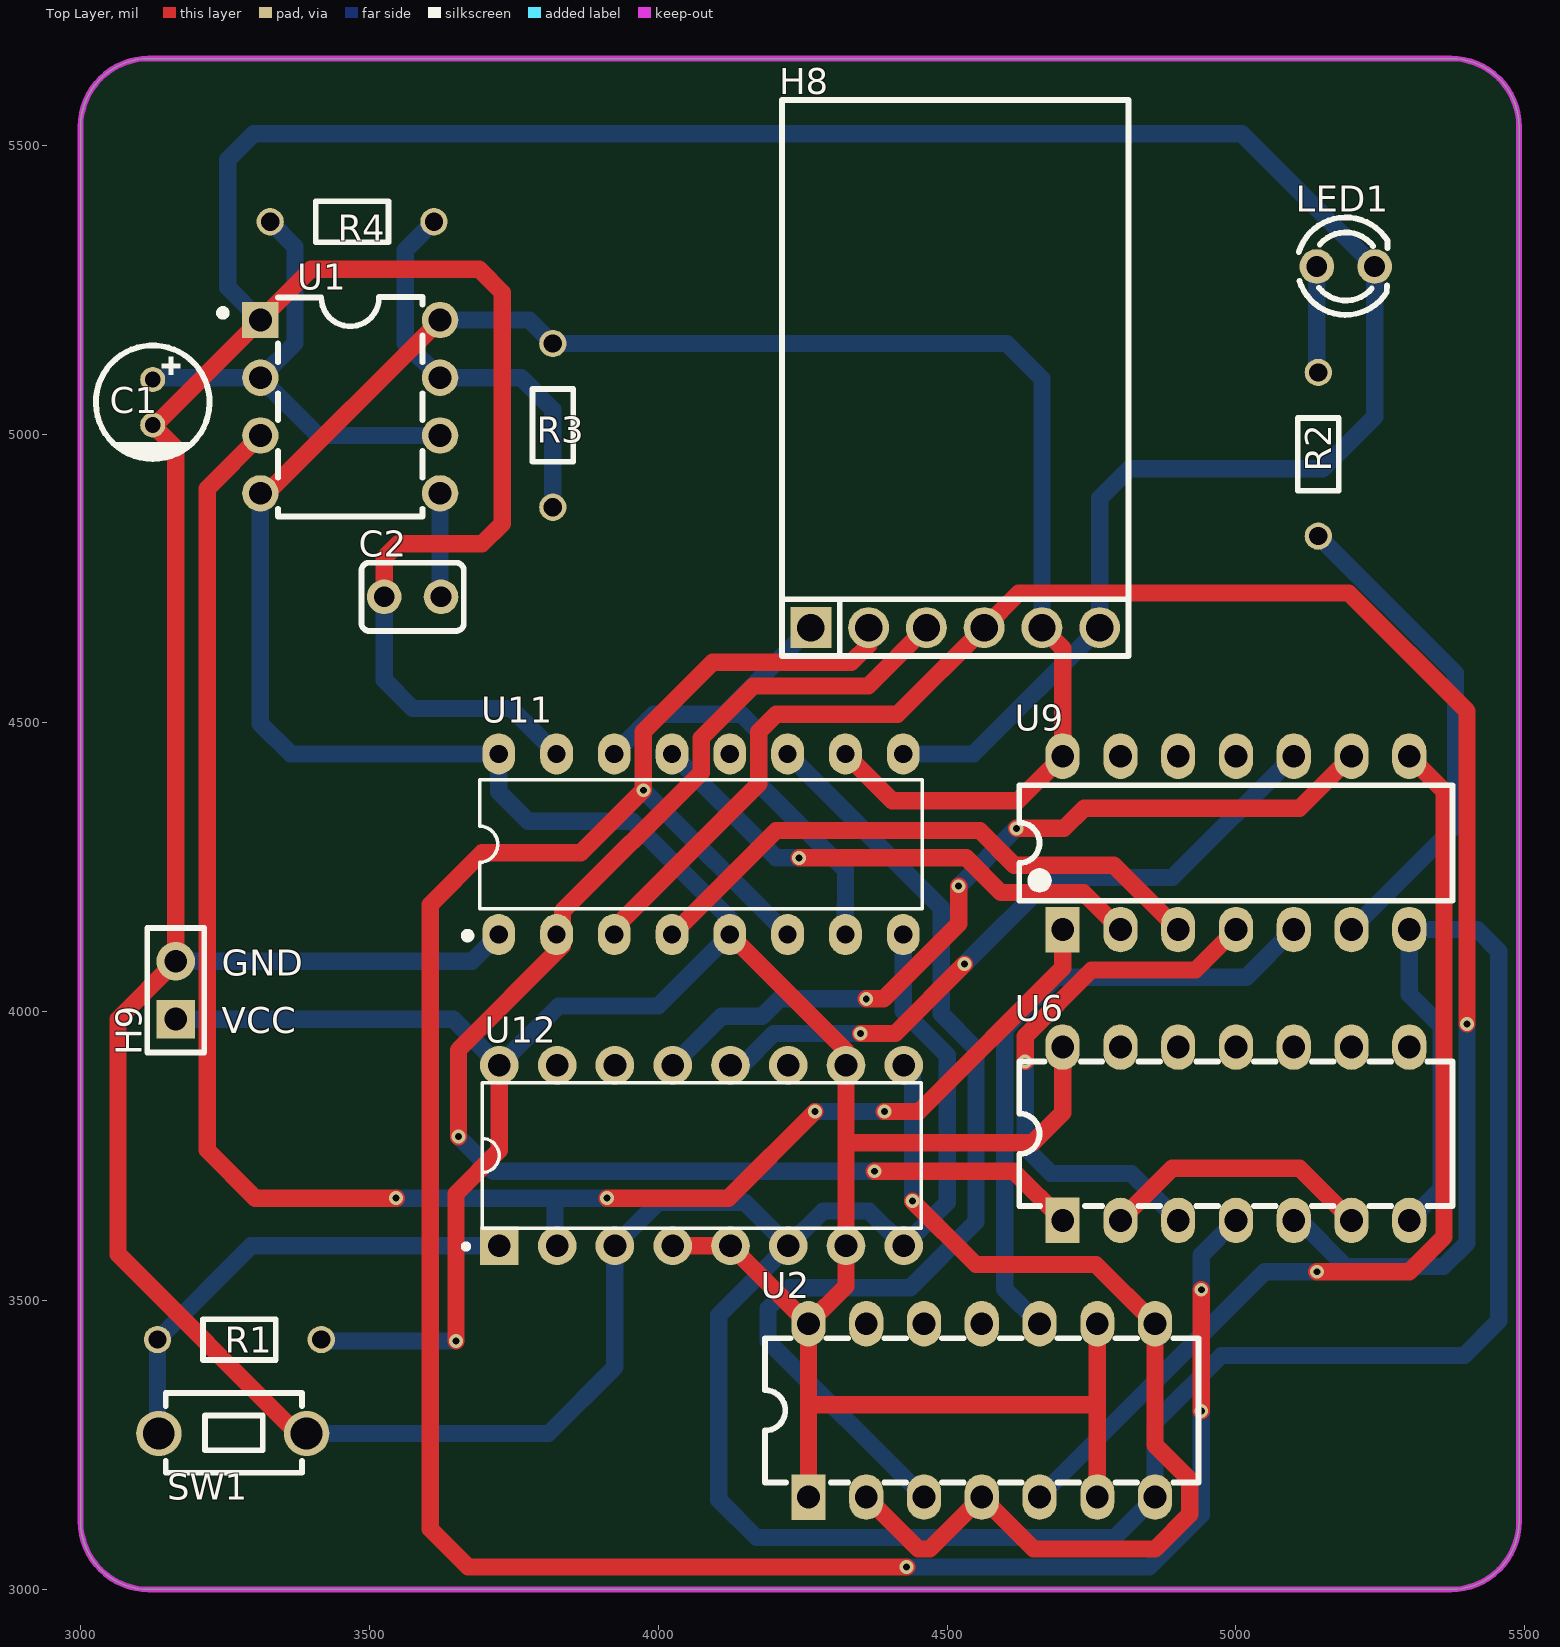
[diagram p0: Top Layer view]
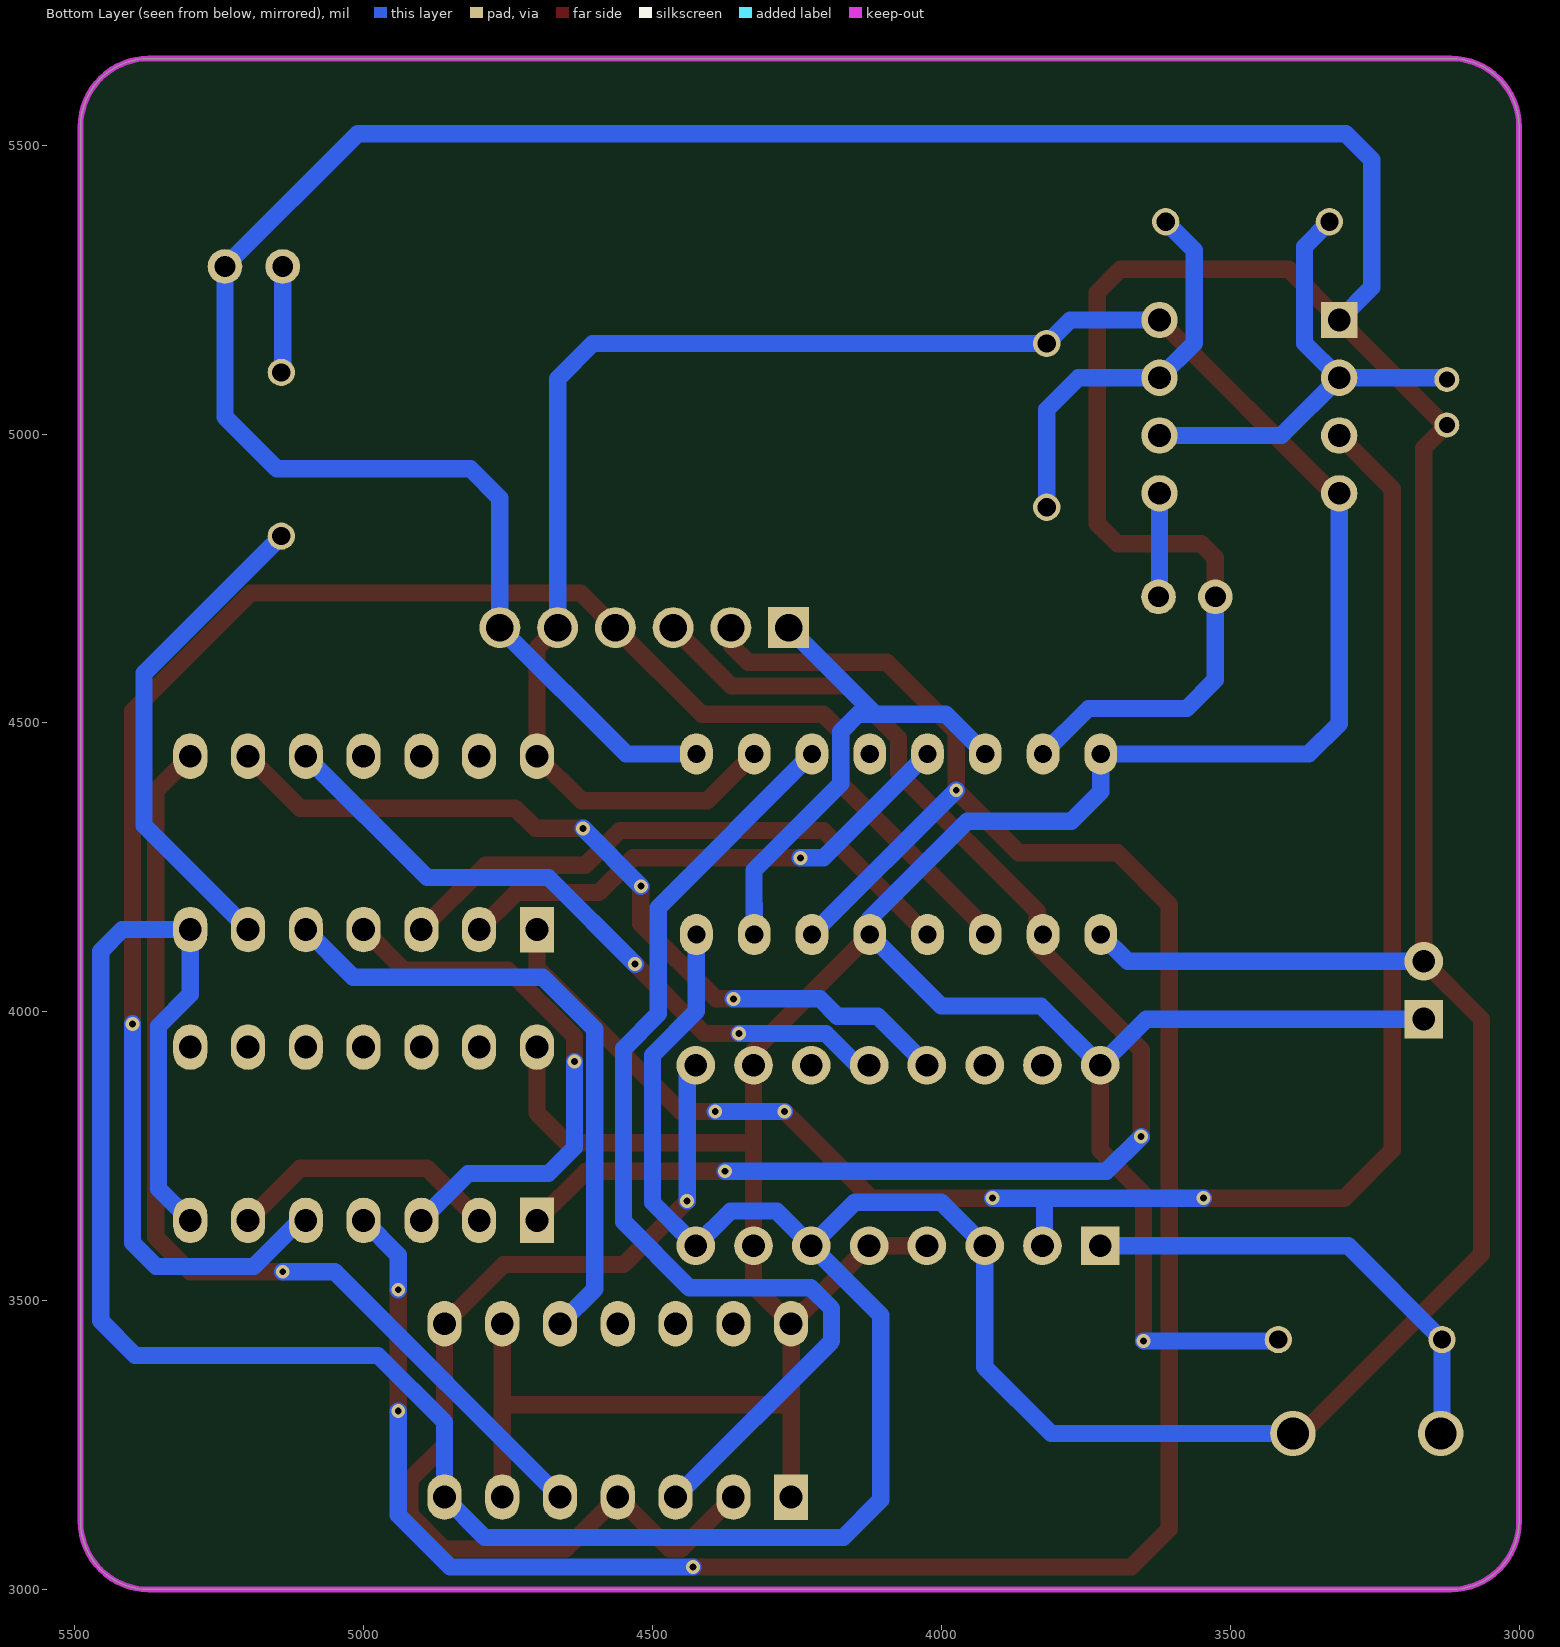
[diagram p1: Bottom Layer view, seen from below]
# Altium PCB MISC51493.pcbdoc
Units mil, origin at the board's own origin, x right, y up, seen from the top; angles counter-clockwise.
Board outline 2490 x 2650 mil, 2 copper layers (Top Layer, Bottom Layer), stack 62.206 mil thick; 16 components, 23 nets, 106 pads, 21 vias.

## Layer stack, top to bottom
Top Solder Mask Layer: solder mask 0.394, Dk 3.3
Top Layer: signal copper 1.379
Dielectric1: surface 59.449, FR4, Dk 4.5
Bottom Layer: signal copper 1.378
Bottom Solder Mask Layer: solder mask 0.394, Dk 3.3

## Board outline
3118.11,5650 ccw(c3118.11,5531.89) 3000,5531.89 3000,3118.11 ccw(c3118.11,3118.11) 3118.11,3000 5371.89,3000 ccw(c5371.89,3118.11) 5490,3118.11 5490,5531.89 ccw(c5371.89,5531.89) 5371.89,5650

## Design rules (kind name [scope] priority, off if disabled: settings)
BoardOutlineClearance copperThickness2oz_1 [All] p2 off: genericclearance=8 ignorepadtopadclearanceinfootprint=FALSE except(0: Arc-SplitContinuation Track-SplitContinuation SMDPad-SplitContinuation THPad-SplitContinuation Via-SplitContinuation Fill-SplitContinuation Region-SplitContinuation Poly-SplitContinuation Text-SplitContinuation Hole-SplitContinuation; 6: Arc-CutoutEdge Track-CutoutEdge SMDPad-CutoutEdge THPad-CutoutEdge Via-CutoutEdge Text-CutoutEdge; 6.9: Hole-OutlineEdge Hole-CutoutEdge; 10: Poly-OutlineEdge Poly-CutoutEdge; 11.8: Arc-OutlineEdge Track-OutlineEdge SMDPad-OutlineEdge THPad-OutlineEdge Via-OutlineEdge Fill-OutlineEdge Region-OutlineEdge Text-OutlineEdge Fill-CutoutEdge Region-CutoutEdge)
BoardOutlineClearance Plane_innerPlane_1 [All] p4 off: genericclearance=4 ignorepadtopadclearanceinfootprint=FALSE except(0: Arc-SplitContinuation Track-SplitContinuation SMDPad-SplitContinuation THPad-SplitContinuation Via-SplitContinuation Fill-SplitContinuation Region-SplitContinuation Poly-SplitContinuation Text-SplitContinuation Hole-SplitContinuation; 6: Arc-CutoutEdge Track-CutoutEdge SMDPad-CutoutEdge THPad-CutoutEdge Via-CutoutEdge Text-CutoutEdge; 6.9: Hole-OutlineEdge Hole-CutoutEdge; 10: Poly-OutlineEdge Poly-CutoutEdge; 11.8: Arc-OutlineEdge Track-OutlineEdge SMDPad-OutlineEdge THPad-OutlineEdge Via-OutlineEdge Fill-OutlineEdge Region-OutlineEdge Text-OutlineEdge Fill-CutoutEdge Region-CutoutEdge)
BoardOutlineClearance Copper_copperRegion_1 [All] p6 off: genericclearance=4 ignorepadtopadclearanceinfootprint=FALSE except(0: Arc-SplitContinuation Track-SplitContinuation SMDPad-SplitContinuation THPad-SplitContinuation Via-SplitContinuation Fill-SplitContinuation Region-SplitContinuation Poly-SplitContinuation Text-SplitContinuation Hole-SplitContinuation; 6: Arc-CutoutEdge Track-CutoutEdge SMDPad-CutoutEdge THPad-CutoutEdge Via-CutoutEdge Text-CutoutEdge; 6.9: Hole-OutlineEdge Hole-CutoutEdge; 10: Poly-OutlineEdge Poly-CutoutEdge; 11.8: Arc-OutlineEdge Track-OutlineEdge SMDPad-OutlineEdge THPad-OutlineEdge Via-OutlineEdge Fill-OutlineEdge Region-OutlineEdge Text-OutlineEdge Fill-CutoutEdge Region-CutoutEdge)
BoardOutlineClearance copperThickness1oz_1 [All] p8: genericclearance=4 ignorepadtopadclearanceinfootprint=FALSE except(0: Arc-SplitContinuation Track-SplitContinuation SMDPad-SplitContinuation THPad-SplitContinuation Via-SplitContinuation Fill-SplitContinuation Region-SplitContinuation Poly-SplitContinuation Text-SplitContinuation Hole-SplitContinuation; 6: Arc-CutoutEdge Track-CutoutEdge SMDPad-CutoutEdge THPad-CutoutEdge Via-CutoutEdge Text-CutoutEdge; 6.9: Hole-OutlineEdge Hole-CutoutEdge; 10: Poly-OutlineEdge Poly-CutoutEdge; 11.8: Arc-OutlineEdge Track-OutlineEdge SMDPad-OutlineEdge THPad-OutlineEdge Via-OutlineEdge Fill-OutlineEdge Region-OutlineEdge Text-OutlineEdge Fill-CutoutEdge Region-CutoutEdge)
Clearance copperThickness2oz [All] p1 off: gap=8 ignorepadtopadclearanceinfootprint=FALSE except(6: SMDPad-Track SMDPad-SMDPad THPad-Track SMDPad-THPad THPad-THPad Track-Via SMDPad-Via THPad-Via Via-Via Fill-SMDPad Region-SMDPad Fill-THPad Region-THPad Fill-Via Region-Via Fill-Fill Fill-Region Region-Region Arc-Track Arc-SMDPad Arc-THPad Arc-Via Fill-Arc Region-Arc Arc-Arc Text-Track SMDPad-Text Text-THPad Text-Via Fill-Text Region-Text Arc-Text Text-Text; 6.9: Hole-Track Hole-SMDPad Hole-THPad Hole-Via Fill-Hole Region-Hole Hole-Arc Hole-Text; 10: Poly-Track Poly-SMDPad Poly-THPad Poly-Via Poly-Fill Poly-Region Poly-Poly Poly-Arc Poly-Text Poly-Hole; 11.8: Fill-Track Region-Track)
Clearance Plane_innerPlane [All] p3 off: gap=4 ignorepadtopadclearanceinfootprint=FALSE except(6: SMDPad-Track SMDPad-SMDPad THPad-Track SMDPad-THPad THPad-THPad Track-Via SMDPad-Via THPad-Via Via-Via Fill-SMDPad Region-SMDPad Fill-THPad Region-THPad Fill-Via Region-Via Fill-Fill Fill-Region Region-Region Arc-Track Arc-SMDPad Arc-THPad Arc-Via Fill-Arc Region-Arc Arc-Arc Text-Track SMDPad-Text Text-THPad Text-Via Fill-Text Region-Text Arc-Text Text-Text; 6.9: Hole-Track Hole-SMDPad Hole-THPad Hole-Via Fill-Hole Region-Hole Hole-Arc Hole-Text; 10: Poly-Track Poly-SMDPad Poly-THPad Poly-Via Poly-Fill Poly-Region Poly-Poly Poly-Arc Poly-Text Poly-Hole; 11.8: Fill-Track Region-Track)
Clearance Copper_copperRegion [All] p5 off: gap=4 ignorepadtopadclearanceinfootprint=FALSE except(6: SMDPad-Track SMDPad-SMDPad THPad-Track SMDPad-THPad THPad-THPad Track-Via SMDPad-Via THPad-Via Via-Via Fill-SMDPad Region-SMDPad Fill-THPad Region-THPad Fill-Via Region-Via Fill-Fill Fill-Region Region-Region Arc-Track Arc-SMDPad Arc-THPad Arc-Via Fill-Arc Region-Arc Arc-Arc Text-Track SMDPad-Text Text-THPad Text-Via Fill-Text Region-Text Arc-Text Text-Text; 6.9: Hole-Track Hole-SMDPad Hole-THPad Hole-Via Fill-Hole Region-Hole Hole-Arc Hole-Text; 10: Poly-Track Poly-SMDPad Poly-THPad Poly-Via Poly-Fill Poly-Region Poly-Poly Poly-Arc Poly-Text Poly-Hole; 11.8: Fill-Track Region-Track)
Clearance copperThickness1oz [All] p7: gap=4 ignorepadtopadclearanceinfootprint=FALSE except(6: SMDPad-Track SMDPad-SMDPad THPad-Track SMDPad-THPad THPad-THPad Track-Via SMDPad-Via THPad-Via Via-Via Fill-SMDPad Region-SMDPad Fill-THPad Region-THPad Fill-Via Region-Via Fill-Fill Fill-Region Region-Region Arc-Track Arc-SMDPad Arc-THPad Arc-Via Fill-Arc Region-Arc Arc-Arc Text-Track SMDPad-Text Text-THPad Text-Via Fill-Text Region-Text Arc-Text Text-Text; 6.9: Hole-Track Hole-SMDPad Hole-THPad Hole-Via Fill-Hole Region-Hole Hole-Arc Hole-Text; 10: Poly-Track Poly-SMDPad Poly-THPad Poly-Via Poly-Fill Poly-Region Poly-Poly Poly-Arc Poly-Text Poly-Hole; 11.8: Fill-Track Region-Track)
DiffPairsRouting differentialPair [All] p1: maxlimit=6 minlimit=6 mostfreqgap=6 toplayer_minwidth=5 toplayer_prefwidth=10 toplayer_maxwidth=100 toplayer_mingap=6 toplayer_prefgap=6 toplayer_maxgap=6 bottomlayer_minwidth=5 bottomlayer_prefwidth=10 bottomlayer_maxwidth=100 bottomlayer_mingap=6 bottomlayer_prefgap=6 bottomlayer_maxgap=6 maxuncoupledlength=10
HoleToHoleClearance otherClearance [All] p1: gap=11.8 allowstackedmicrovias=TRUE
Length netLength [All] p1: minlimit=0 maxlimit=0
PasteMaskExpansion pasteMaskExpansion [All] p1: expansion=0
PlaneConnect innerPlane [All] p1: planeconnectstyle=Relief reliefexpansion=20 reliefentries=4 reliefconductorwidth=10 reliefairgap=10
PolygonConnect copperRegion [All] p1: connectstyle=Relief reliefconductorwidth=10 reliefentries=4 polygonreliefangle="90 Angle" airgapwidth=10 via.connectstyle=Relief via.reliefconductorwidth=10 via.reliefentries=4 via.polygonreliefangle="90 Angle" via.airgapwidth=10
RoutingVias viaSize [All] p1: holewidth=12 width=24 viastyle="Through Hole" minholewidth=11.8 minwidth=19.7 maxholewidth=248 maxwidth=393.7
SolderMaskExpansion solderMaskExpansion [IsVia] p1: expansion=-1000 istentingtop=TRUE
SolderMaskExpansion solderMaskExpansion [All] p2: expansion=2 istentingtop=FALSE
Width copperThickness2oz_2 [All] p1 off: maxlimit=100 minlimit=8 preferedwidth=10
Width copperThickness1oz_2 [All] p2: maxlimit=100 minlimit=5 preferedwidth=30

## Components (designator, comment, footprint, x,y, rotation, side; value= is the part's Value field where it differs from the comment)
C1 "10uF" CAP-TH_BD5.0-P2.00-D0.5-FD 3125,5055 r270 top
C2 "100nF" CAP-TH_L4.5-W3.0-P2.50-D0.5 3574.86,4718.21 r0 top
H8 "" HDR-TH_6P-P2.54-V-M-1 4514.18,4664.82 r0 top
H9 "" HDR-TH_2P-P2.54-V-F 3164.86,4037.31 r90 top
LED1 "" LED_TH-3mm 5190,5290 r0 top
R1 "10kΩ" Res_1/8W 3275,3435 r180 top
R2 "300Ω" Res_1/8W 5140,4965 r270 top
R3 "47kΩ" Res_1/8W 3820,5015 r90 top
R4 "47kΩ" Res_1/8W 3470,5365 r0 top
SW1 "" Key_TH_3.5x6x4.3 3270,3270 r180 top
U1 "NE555PE4" PDIP-8_L9.6-W6.4-P2.54-LS7.9-BL-1 3466.84,5047.41 r270 top
U2 "SN74HC266N" PDIP-14_L19.3-W6.4-P2.54-LS7.6-BL 4560,3310 r0 top
U6 "CD74HC32EG4" PDIP-14_L19.3-W6.4-P2.54-LS7.6-BL 5000,3788.84 r0 top
U9 "74HC08DN" PDIP-14_L19.3-W6.5-P2.54-LS7.6-BL 5000,4292.36 r0 top
U11 "74LS192D" PDIP-16_L19.3-W6.4-P2.54-LS7.94-BL 4073.95,4290 r0 top
U12 "SN74HC161NG4" PDIP-16_L19.3-W6.4-P2.54-LS7.9-BL 4075,3751.16 r0 top

## Footprints (in the part's own frame and the unit in brackets; to place one, negate y for a bottom-side part, rotate by r counter-clockwise, add the part's x,y. Pads: shape width x height; smd on the part's side, far side on the other; paste and mask are expansions set on the pad)
CAP-TH_BD5.0-P2.00-D0.5-FD [mm]
  round 1.1 hole 0.7 paste+0 mask+0.05: 1(-1,0) 2(1,0)
  silkscreen extent -2.5,-2.5 2.5,2.5
CAP-TH_L4.5-W3.0-P2.50-D0.5 [mil]
  round 60 hole 36 paste+0 mask+1.97: 1(-49.21,0) 2(49.21,0)
  silkscreen extent -89,-59 89,59
HDR-TH_2P-P2.54-V-F [mm]
  rect 1.7x1.7 hole 1: 1(-1.27,0)
  round 1.7 hole 1: 2(1.27,0)
  silkscreen extent -2.74,-1.25 2.74,1.25
HDR-TH_6P-P2.54-V-M-1 [mm]
  rect 1.8x1.8 hole 1.2: 1(-6.35,0)
  round 1.8 hole 1.2: 2(-3.81,0) 3(-1.27,0) 4(1.27,0) 5(3.81,0) 6(6.35,0)
  silkscreen extent -7.62,-1.25 7.62,23.2
Key_TH_3.5x6x4.3 [mil]
  round 78.7 hole 55.1 paste+0 mask+2: A(-121.44,0) B(134.46,0)
  silkscreen extent -114,-70 123,68
LED_TH-3mm [mil]
  round 60 hole 36 paste+0 mask+2: 1(-50,0) 2(50,0)
  silkscreen extent -81,-84 72,85
PDIP-8_L9.6-W6.4-P2.54-LS7.9-BL-1 [mil]
  rect 63x63 hole 39.37: 1(-150,-155.51)
  round 63 hole 39.37: 2(-50,-155.51) 3(50,-155.51) 4(150,-155.51) 5(150,155.52) 6(50,155.52) 7(-50,155.52) 8(-150,155.52)
  silkscreen extent -190,-226 190,125
PDIP-14_L19.3-W6.4-P2.54-LS7.6-BL [mm]
  rect 1.5x2 hole 1: 1(-7.62,-3.81)
  oval 1.5x2 hole 1: 2(-5.08,-3.81) 3(-2.54,-3.81) 4(0,-3.81) 5(2.54,-3.81) 6(5.08,-3.81) 7(7.62,-3.81) 8(7.62,3.81) 9(5.08,3.81) 10(2.54,3.81) 11(0,3.81) 12(-2.54,3.81) 13(-5.08,3.81) 14(-7.62,3.81)
  silkscreen extent -9.53,-3.17 9.53,3.17
PDIP-14_L19.3-W6.5-P2.54-LS7.6-BL [mm]
  rect 1.5x2 hole 1: 1(-7.62,-3.81)
  oval 1.5x2 hole 1: 2(-5.08,-3.81) 3(-2.54,-3.81) 4(0,-3.81) 5(2.54,-3.81) 6(5.08,-3.81) 7(7.62,-3.81) 8(7.62,3.81) 9(5.08,3.81) 10(2.54,3.81) 11(0,3.81) 12(-2.54,3.81) 13(-5.08,3.81) 14(-7.62,3.81)
  silkscreen extent -9.53,-2.55 9.53,2.53
PDIP-16_L19.3-W6.4-P2.54-LS7.9-BL [mm]
  rect 1.7x1.7 hole 1: 1(-8.89,-3.97)
  round 1.7 hole 1 copper offset 0,0: 2(-6.35,-3.97) 3(-3.81,-3.97) 4(-1.27,-3.97) 5(1.27,-3.97) 6(3.81,-3.97) 7(6.35,-3.97) 8(8.89,-3.97)
  round 1.7 hole 1: 9(8.89,3.97) 10(6.35,3.97) 11(3.81,3.97) 12(1.27,3.97) 13(-1.27,3.97) 14(-3.81,3.97) 15(-6.35,3.97) 16(-8.89,3.97)
  silkscreen extent -10.46,-4.1 9.65,3.2
PDIP-16_L19.3-W6.4-P2.54-LS7.94-BL [mm]
  oval 1.44x1.8 hole 0.8: 1(-8.89,-3.97) 2(-6.35,-3.97) 3(-3.81,-3.97) 4(-1.27,-3.97) 5(1.27,-3.97) 6(3.81,-3.97) 7(6.35,-3.97) 8(8.89,-3.97) 9(8.89,3.97) 10(6.35,3.97) 11(3.81,3.97) 12(1.27,3.97) 13(-1.27,3.97) 14(-3.81,3.97) 15(-6.35,3.97) 16(-8.89,3.97)
  silkscreen extent -10.41,-4.17 9.73,2.84
Res_1/8W [mil]
  round 47.2 hole 31.5 paste+0 mask+2: 1(-141.7,2.48) 2(141.7,2.48)
  silkscreen extent -63,-33 63,38

## Via types
v1: diameter 24, hole 12, Top Layer to Bottom Layer, 20 vias
v2: diameter 24.02, hole 12, Top Layer to Bottom Layer, 1 vias

## Nets (pads, with @x,y where several pads share a name; then routed paths per layer and width w, separated by ;. In a path a pad name is that pad's centre, name@x,y a point inside that pad or via, vN(x,y) a via of type N, cw(c..) or ccw(c..) an arc to the next point about the centre after c; other vN are vias at no path point)
$1N282: R3.1 R4.2 U1.7 | length 702.5
  Bottom Layer w30: R4.2 3562.35,5318.12 3562.35,5157.41 3622.35,5097.41 3762.59,5097.41 3817.52,5042.48 R3.1
$1N283: C1.1 R4.1 U1.2 U1.6 | length 852.8
  Bottom Layer w30: C1.1 3128.04,5097.41 U1.2 ; R4.1 3371.33,5324.45 3371.33,5157.41 U1.2 ; U1.6@3622.35,4997.41 3411.33,4997.41 U1.2
$1N284: C2.2 U1.5 | length 179.9
  Bottom Layer w30: U1.5@3622.35,4897.41 3622.35,4719.94 C2.2
$1N3868: R1.2 SW1.B U12.1 | length 822.4
  Bottom Layer w30: SW1.B 3133.3,3272.24 R1.2 3295.64,3594.86 U12.1
$1N5236: LED1.1 R2.1 | length 184.3
  Bottom Layer w30: LED1.1 5140,5109.18 R2.1
DCDA: H8.1 U11.7 U11.14 | length 916.4
  Bottom Layer w30: U11.14 3992.46,4514.82 4114.18,4514.82 ; H8.1 4114.18,4514.82 ; U11.7 4324.18,4244.82 4174.18,4394.82 4174.18,4484.82 4144.18,4514.82 4114.18,4514.82
DCDB: H8.2 U6.4 U11.6 | length 4402.4
  Top Layer w30: H8.2 4364.18,4634.82 4334.18,4604.82 4094.18,4604.82 3974.18,4484.82 v1(3974.18,4383.47) 3865.71,4275 3695,4275 3605.33,4185.33 3605.33,3104.67 3671.16,3038.84 v1(4430,3038.84) ; v1(4940,3308.84) v1(4940,3518.84)
  Bottom Layer w30: v1(3974.18,4383.47) U11.6 ; v1(4430,3038.84) 4850,3038.84 4940,3128.84 v1(4940,3308.84) ; v1(4940,3518.84) 4940,3578.84 U6.4
DCDC: H8.3 U6.1 U11.2 | length 2453.4
  Top Layer w30: v1(3654.18,3783.93) 3654.18,3933.93 3834.18,4113.93 U11.2@3834.18,4143.93 ; U11.2 U11.2@3834.18,4143.93 ; v1(4374.18,3723.93) 4614.9,3723.93 U6.1 ; H8.3 4363.3,4563.93 4164.18,4563.93 4074.18,4473.93 4074.18,4413.93 3834.18,4173.93 U11.2@3834.18,4143.93
  Bottom Layer w30: v1(3654.18,3783.93) 3714.18,3723.93 v1(4374.18,3723.93)
DCDD: H8.4 U6.5 U11.3 | length 3134.9
  Top Layer w30: U11.3 3923.95,4144.58 4174.18,4394.82 4174.18,4484.82 4204.18,4514.82 4414.18,4514.82 H8.4 4624.18,4724.82 5195.18,4724.82 5400,4520 v1(5400,3979)
  Bottom Layer w30: U6.5 5110.16,3638.84 5190,3559 5359,3559 5400,3600 v1(5400,3979)
GND: C1.2 C2.1 H8.6 H9.2 LED1.2 SW1.A U1.1 U2.7 U6.7 U9.7 U11.1 U11.8 U11.9 U11.15 U12.3 U12.6 U12.8 | length 13762.5
  Top Layer w30: SW1.A 3375,3270 3065,3580 3065,3987.45 H9.2 3164.86,4975.77 C1.2 3129.54,5015.63 U1.1 3398.91,5285 3690,5285 3730,5245 3730,4845 3695,4810 3550,4810 3525.65,4785.65 C2.1
  Bottom Layer w30: H9.2 3677.55,4087.31 U11.1 ; U1.1 3255,5253.74 3255,5475 3300,5520 5010,5520 LED1.2 5240,5030 5150,4940 4815,4940 4764.18,4889.18 H8.6 4545.66,4446.3 U11.9 ; SW1.A 3810,3270 3925,3385 U12.3 4000.14,3670 4149.86,3670 U12.6 ; C2.1 3525.65,4574.35 3575,4525 3745.25,4525 U11.15 ; U11.8 4423.95,4001.05 4500,3925 4500,3669.86 U12.8 4364.86,3655 4285.14,3655 U12.6 ; U6.7 5355,3693.84 5355,3975 5300,4030 U9.7 5417.64,4142.36 5455,4105 5455,3465 5395,3405 4975,3405 4860,3290 U2.7 4790,3090 4170,3090 4105,3155 4105,3474.86 U12.6
NE555OUT: U1.3 U9.1 U12.2 | length 3105.5
  Top Layer w30: U1.3 3219.33,4905.41 3219.33,3760.67 3302.59,3677.41 v1(3546.33,3677.41) ; v1(3911.33,3677.41) 4121.33,3677.41 v1(4271.33,3827.41) ; v1(4391.33,3827.41) 4451.33,3827.41 4700,4076.09 U9.1
  Bottom Layer w30: v1(3546.33,3677.41) 3821.33,3677.41 ; U12.2 3821.33,3598.53 3821.33,3677.41 ; v1(3911.33,3677.41) 3821.33,3677.41 ; v1(4271.33,3827.41) v1(4391.33,3827.41)
U2A3: U2.3 U11.11 | length 1805.3
  Bottom Layer w30: U11.11 4490,4180.25 4490,3996.3 4550,3936.3 4550,3636.3 4436,3522.3 4226,3522.3 4190,3486.3 4190,3430 U2.3
U4A1: U6.3 U9.4 | length 951.3
  Top Layer w30: v1(4635,3913.84) 4635,3957.36 4750,4072.36 4930,4072.36 U9.4
  Bottom Layer w30: v1(4635,3913.84) 4635,3765 4680,3720 4818.84,3720 U6.3
U4A3: R2.2 U9.6 | length 853.9
  Bottom Layer w30: R2.2 5380,4585.78 5380,4322.36 U9.6
U6A2: U9.2 U11.13 | length 901.9
  Top Layer w30: v1(4243.95,4266.3) 4533.26,4266.3 4593.26,4206.3 4736.06,4206.3 U9.2
  Bottom Layer w30: U11.13 4203.95,4266.3 v1(4243.95,4266.3)
U6A3: U9.3 U11.4 | length 1021.6
  Top Layer w30: U11.4 4203.95,4313.7 4556.3,4313.7 4616.3,4253.7 4788.66,4253.7 U9.3
U10A3: U6.2 U6.6 | length 474.6
  Top Layer w30: U6.2 4890,3728.84 5110,3728.84 U6.6
U11A2: U2.2 U2.4 U2.8 U12.9 | length 1800.8
  Top Layer w30: U2.2 4450,3070 4470,3070 U2.4 4650,3070 4860,3070 4920,3130 4920,3190 4860,3250 U2.8 4757.54,3562.46 4550,3562.46 v1(4440,3672.46)
  Bottom Layer w30: U12.9 4440,3892.46 v1(4440,3672.46)
U11A3: U2.10 U9.5 | length 1106.2
  Bottom Layer w30: U2.10 4600,3520 4600,3970 4690,4060 5017.64,4060 U9.5
U12A2: U2.5 U9.8 | length 1743.6
  Top Layer w30: v1(5140,3550) 5300,3550 5360,3610 5360,4382.36 U9.8
  Bottom Layer w30: U2.5 5050,3550 v1(5140,3550)
U13A1: U9.9 U12.13 | length 1434.6
  Top Layer w30: v1(4360,4022.36) 4390,4022.36 4520,4152.36 v1(4520,4217.36) ; v1(4620,4317.36) 4702.36,4317.36 4737.36,4352.36 5110,4352.36 U9.9
  Bottom Layer w30: U12.13 4109.9,3992.36 4180,3992.36 4210,4022.36 v1(4360,4022.36) ; v1(4520,4217.36) v1(4620,4317.36)
U13A2: U9.10 U12.12 | length 1196.6
  Top Layer w30: v1(4350,3962.36) 4410,3962.36 v1(4530,4082.36)
  Bottom Layer w30: U12.12 4145.1,3907.46 4200,3962.36 v1(4350,3962.36) ; v1(4530,4082.36) 4680,4232.36 4890,4232.36 U9.10
VCC: H8.5 H9.1 R1.1 R3.2 U1.4 U1.8 U2.1 U2.6 U2.9 U2.14 U6.14 U9.14 U11.5 U11.10 U11.16 U12.4 U12.5 U12.7 U12.10 U12.16 | length 8560.3
  Top Layer w30: U1.4 3322.35,4897.41 U1.8@3622.35,5197.41 ; v2(3650,3430) 3650,3685 3725,3760 U12.16 ; U12.4 U12.5 4259.86,3460 U2.14 ; U11.5 4325,3932.65 U12.10 4325,3773.4 ; U2.1 4260,3319.88 ; U11.10 4405.25,4365 4622.64,4365 U9.14 4700,4629 H8.5 ; U6.14 4700,3825 4648.4,3773.4 4325,3773.4 ; U2.6 4760,3318.68 ; U2.9 4760,3318.68 ; 4260,3319.88 4758.8,3319.88 4760,3318.68 ; 4260,3319.88 U2.14 ; U2.14 4325,3525 U12.7 4325,3773.4
  Bottom Layer w30: H9.1 3645.15,3987.31 U12.16 3827.54,4010 4000.25,4010 U11.5 4123.95,4161.05 3955,4330 3775,4330 3723.95,4381.05 U11.16 3363.7,4446.3 3311.33,4498.67 U1.4 ; R1.1 3419.22,3430 v2(3650,3430) ; U1.8@3622.35,5197.41 3776.81,5197.41 R3.2 4603.3,5156.7 4664.18,5095.82 H8.5
pads on no net: U2.11 U2.12 U2.13 U6.8 U6.9 U6.10 U6.11 U6.12 U6.13 U9.11 U9.12 U9.13 U11.12 U12.11 U12.14 U12.15

## Keep-outs
Board Outline Layer:
  the board outline again, w10

## Silkscreen, mask and mechanical layers (free items; w line width, h text height)
Top Silkscreen Layer:
  text "GND" at 3244.6,4062.5 h45
  text "VCC" at 3244.6,3962.5 h45